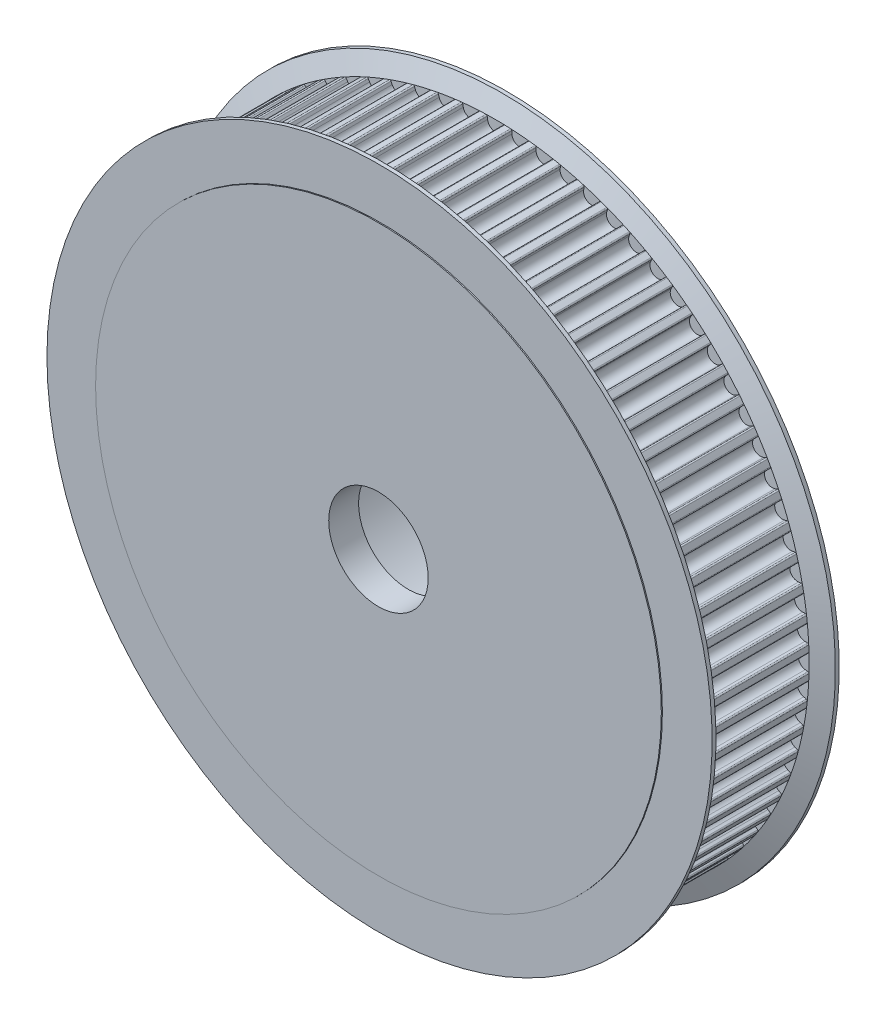
from build123d import *

# Parameters (mm, degrees)
CUT_EXTRUDE_START        = 2.5
CUT_EXTRUDE_2_DEPTH      = 21
PATTERN_CIRCULAR_1_COUNT = 80
SKETCH_9_R               = 23.5
CUT_EXTRUDE_3_DEPTH      = 20
SKETCH_10_R              = 10
CUT_EXTRUDE_4_DEPTH      = 10


with BuildPart() as part:
    # 草图1 → 旋转1 (revolve)
    with BuildSketch(Plane(origin=(0, 0, 0), x_dir=(0, 0, -1), z_dir=(1, 0, 0)), mode=Mode.PRIVATE) as revolve_1_sk:
        Polygon((0, 9.5), (-26, 9.5), (-26, 56.8855), (-25.78, 56.8855), (-25.78, 66.8855), (-25.01, 66.8855), (-23.5, 63.1055), (-2.5, 63.1055), (-0.99, 66.8855), (-0.22, 66.8855), (-0.22, 56.8855), (0, 56.8855), align=None)
    revolve(revolve_1_sk.sketch.rotate(Axis((0, 0, 0), (0, 0, 1)), 90), axis=Axis((0, 0, 0), (0, 0, 1)))

    # 草图2 → 切除-拉伸2 (cut)
    with BuildSketch(Plane.XY.offset(CUT_EXTRUDE_START)):
        with BuildLine():
            Line((1.559587191, 62.32530619), (1.625, 62.858050767))
            ThreePointArc((1.625, 62.858050767), (1.710290154, 63.01727016), (1.880586707, 63.077472396))
            ThreePointArc((1.880586707, 63.077472396), (0, 63.1055), (-1.880586707, 63.077472396))
            ThreePointArc((-1.880586707, 63.077472396), (-1.710290154, 63.01727016), (-1.625, 62.858050767))
            Line((-1.625, 62.858050767), (-1.559587191, 62.32530619))
            ThreePointArc((-1.559587191, 62.32530619), (0, 60.9455), (1.559587191, 62.32530619))
        make_face()
    cut_extrude_2 = extrude(amount=CUT_EXTRUDE_2_DEPTH, mode=Mode.SUBTRACT)

    # 阵列(圆周)1: 切除-拉伸2 ×80 about axis
    pattern_circular_1_axis = Axis((0, 0, 0), (0, 0, 1))
    for i in range(1, PATTERN_CIRCULAR_1_COUNT):
        add(cut_extrude_2.rotate(pattern_circular_1_axis, i * 360 / PATTERN_CIRCULAR_1_COUNT), mode=Mode.SUBTRACT)

    # 草图9 → 切除-拉伸3 (cut)
    with BuildSketch(Plane(origin=(0, 0, 0), x_dir=(-1, 0, 0), z_dir=(0, 0, -1))):
        Circle(SKETCH_9_R)
    extrude(amount=-CUT_EXTRUDE_3_DEPTH, mode=Mode.SUBTRACT)

    # 草图10 → 切除-拉伸4 (cut)
    with BuildSketch(Plane(origin=(0, 0, 20), x_dir=(-1, 0, 0), z_dir=(0, 0, -1))):
        Circle(SKETCH_10_R)
    extrude(amount=-CUT_EXTRUDE_4_DEPTH, mode=Mode.SUBTRACT)


solid = part.part
